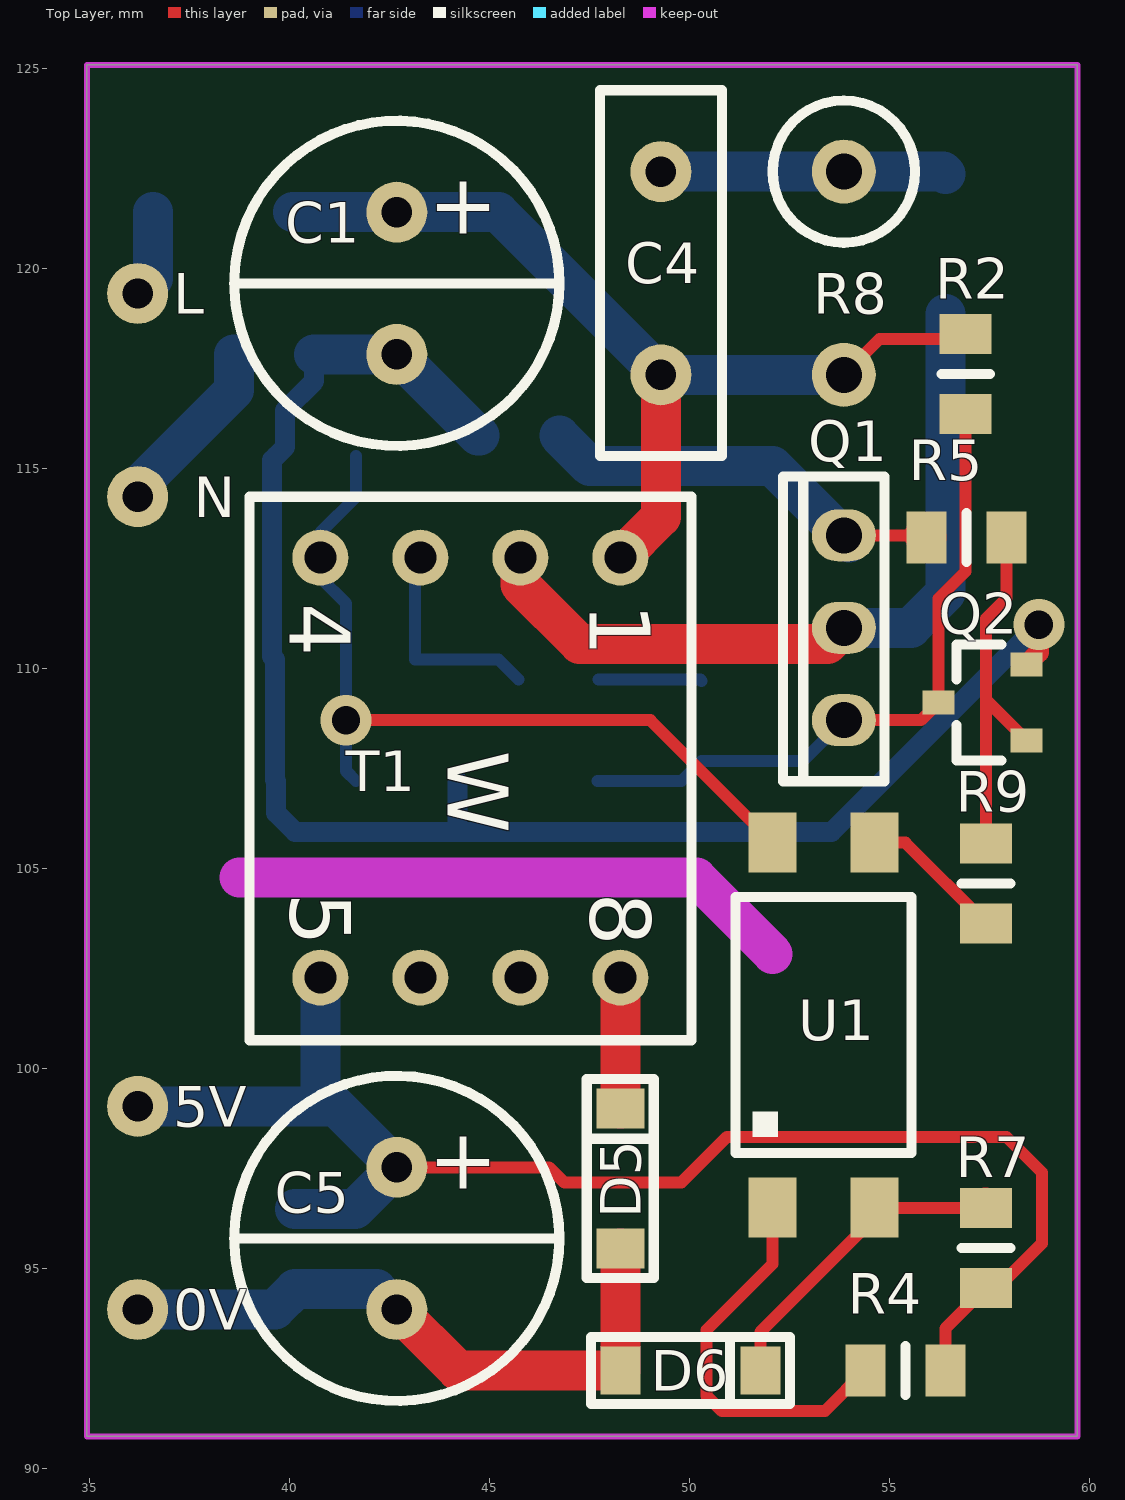
[diagram p0: Top Layer view]
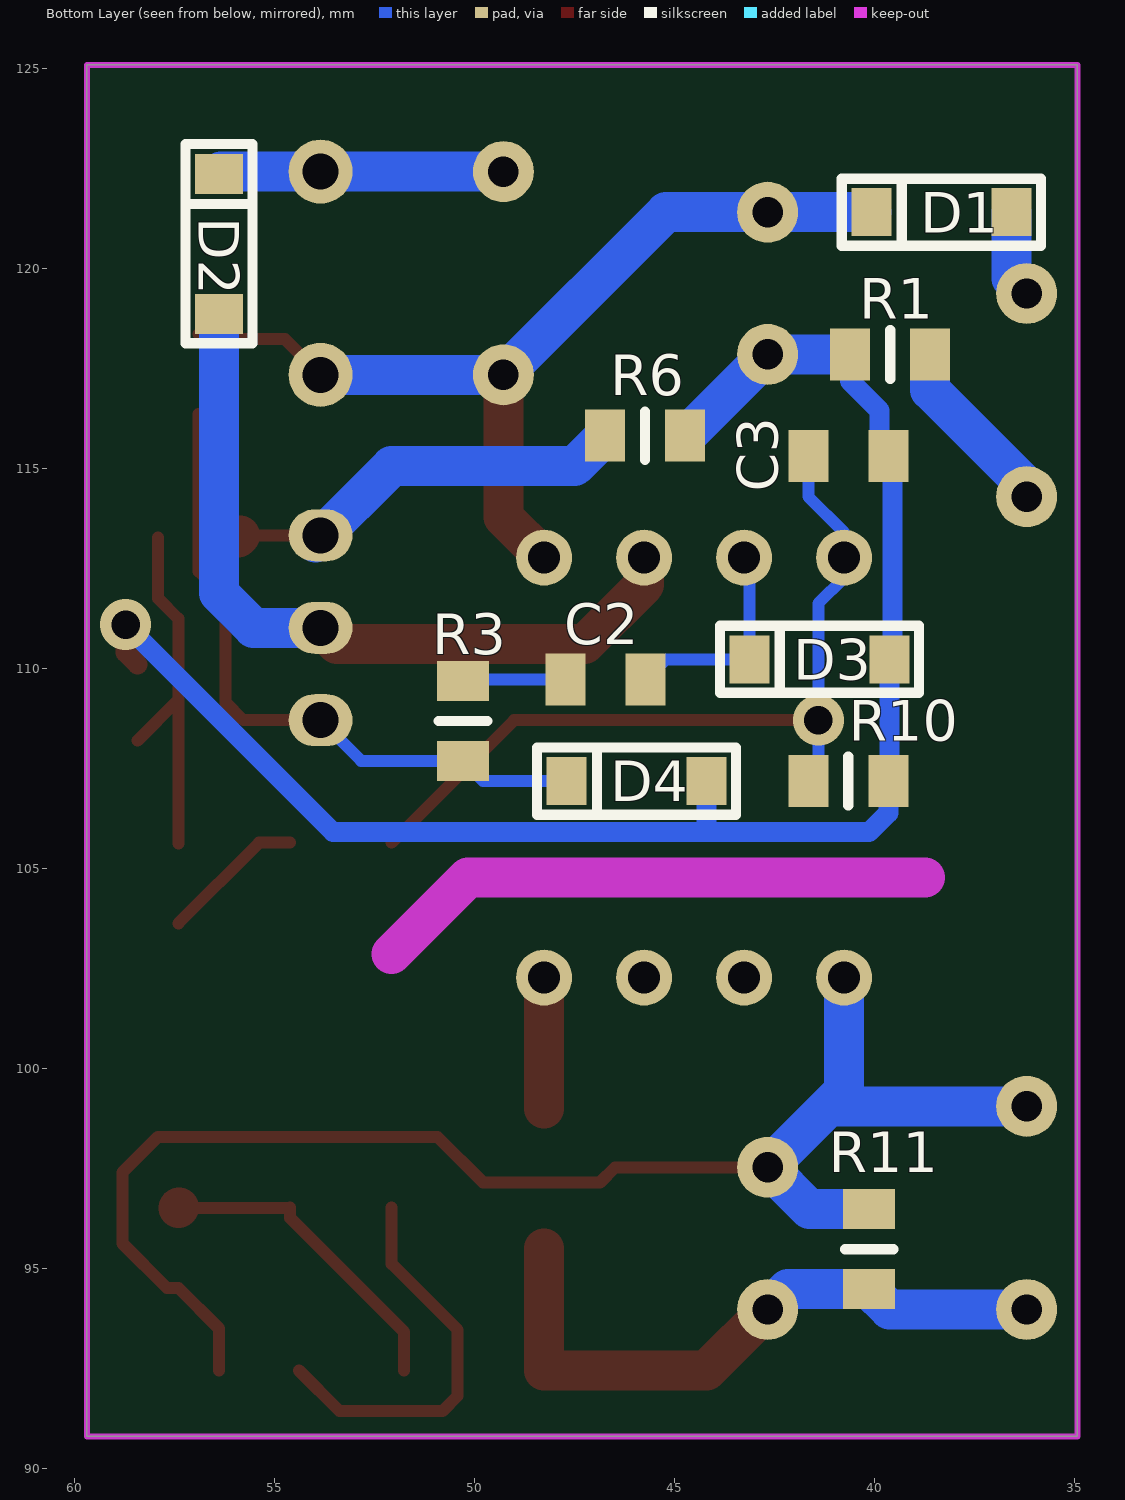
[diagram p1: Bottom Layer view, seen from below]
# Altium PCB MISC95139.PcbDoc
Units mm, origin at the board's own origin, x right, y up, seen from the top; angles counter-clockwise.
Board outline 24.77 x 34.29 mm, 2 copper layers (Top Layer, Bottom Layer); 26 components, 18 nets, 66 pads, 2 vias.

## Layer stack, top to bottom (the 12.6 mil dielectric is the usual default, probably not edited)
Top Layer: signal copper 0.0356
Dielectric: dielectric 0.32, FR-4, Dk 4.8
Bottom Layer: signal copper 0.0356

## Board outline
34.925,125.095 34.925,90.805 59.69,90.805 59.69,125.095

## Design rules (kind name [scope] priority, off if disabled: settings)
Clearance [All] p1: gap=0.254
PolygonConnect [All] p1: connectstyle=Relief reliefconductorwidth=0.254 reliefentries=4 polygonreliefangle="90 Angle"
RoutingVias [All] p1: holewidth=0.711 width=1.27 viastyle="Through Hole" minholewidth=0.711 minwidth=1.27 maxholewidth=0.711 maxwidth=1.27
SilkscreenOverComponentPads [All] p1: minsilkscreentomaskgap=0.254
SolderMaskExpansion [All] p1: expansion=0.102
Width [All] p1: maxlimit=1.5 minlimit=0.3 preferedwidth=1 minimp=50.000000 maximp=50.000000 favimp=50.000000
27 further rules are at their usual default settings.

## Components (designator, comment, footprint, x,y, rotation, side; value= is the part's Value field where it differs from the comment)
C1 "400V4.7uF" cap-8*14mm 42.672,121.412 r270 top
C2 "10nF" 0805_Cap 45.72,109.728 r0 bottom
C3 "16V10uF" 0805_Cap 41.656,115.316 r180 bottom
C4 "1KV4.7nF" CAP_5mm 49.276,117.348 r90 top
C5 "16V470uF" cap-8*14mm 42.672,97.536 r270 top
D1 "1N4007" SOD-123 36.576,121.412 r0 bottom
D2 "FR107" SOD-123 56.388,118.872 r90 bottom
D3 "1N4148" SOD-123 39.624,110.236 r0 bottom
D4 "18V" SOD-123 44.196,107.188 r0 bottom
D5 "B5819W" SOD-123 48.26,95.504 r90 top
D6 "3.9V" SOD-123 48.26,92.456 r0 top
Q1 "1N60" TO-126 53.848,108.712 r90 top
Q2 "J3" SOT23 58.42,108.204 r90 top
R1 "10R" 0805_Res 38.608,117.856 r0 bottom
R2 "2.2M" 0805_Res 56.896,118.364 r270 top
R3 "1K" 0805_Res 50.292,107.696 r90 bottom
R4 "10R" 0805_Res 56.388,92.456 r180 top
R5 "200R" 0805_Res 57.912,113.284 r180 top
R6 "4.7R" 0805_Res 46.736,115.824 r180 bottom
R7 "200R" 0805_Res 57.404,96.52 r270 top
R8 "82K/1W" 1W_Res_L 53.848,122.428 r270 top
R9 "200R" 0805_Res 57.404,103.632 r90 top
R10 "10K" 0805_Res 41.656,107.188 r180 bottom
R11 "1K" 0805_Res 40.132,94.488 r90 bottom
T1 "EE10_4+4_W" EE10_4+4_W 48.26,112.776 r270 top
U1 "PC817" SOP4-PC817 53.34,101.092 r90 top

## Footprints (in the part's own frame and the unit in brackets; to place one, negate y for a bottom-side part, rotate by r counter-clockwise, add the part's x,y. Pads: shape width x height; smd on the part's side, far side on the other; paste and mask are expansions set on the pad)
1W_Res_L [mm]
  round 1.6 hole 0.9: 1(5.08,0) 2(0,0)
  silkscreen extent -1.78,-1.78 1.78,1.78
0805_Cap [mm]
  rect 1x1.3 smd: 1(0,0) 2(2,0)
0805_Res [mm]
  rect 1x1.3 smd: 1(0,0) 2(2,0)
  silkscreen extent 1,-0.61 1,0.61
cap-8*14mm [mil] "470uF/16V,diameter_8mm,height_14mm"
  round 60 hole 30: 1(0,0) 2(140,0)
  silkscreen extent -90,-160 230,160
CAP_5mm [mil] "10nF/1KV,Pin Distance 5mm"
  round 60 hole 30: 1(0,0) 2(200,0)
  silkscreen extent -80,-60 280,60
EE10_4+4_W [mm]
  round 1.4 hole 0.8: 1(0,0) 2(0,-2.5) 3(0,-5) 4(0,-7.5) 5(10.5,-7.5) 6(10.5,-5) 7(10.5,-2.5) 8(10.5,0)
  silkscreen extent -1.52,-9.27 12.07,1.78
SOD-123 [mm]
  rect 1x1.2 smd: 1(0,0) 2(3.5,0)
  silkscreen extent -0.74,-0.84 4.24,0.84
SOP4-PC817 [mm] "SOP4 for PC817"
  rect 1.5x1.2 smd: 1(-4.56,1.27) 2(-4.56,-1.27) 3(4.56,-1.27) 4(4.56,1.27)
  silkscreen extent -3.2,-2.2 3.2,2.2
SOT23 [mm]
  rect 0.6x0.8 smd: 1(0,0) 2(1.9,0) 3(0.95,2.2)
  silkscreen extent -0.5,0.64 2.4,1.75
TO-126 [mm]
  oval 1.3x1.6 hole 0.9: 1(0,0) 2(2.311,0) 3(4.623,0)
  silkscreen extent -1.52,-1.02 6.1,1.52

## Part data
C1 C3 C5: library part "Cap Pol"
C2 C4: library part Cap, "Capacitor"
D1 D2 D3 D5: library part Diode
D4 D6: library part DZener
Q1: library part FQPF20N60C, "600V 20A N-Channel MOSFET"
Q2: "SMD 9013 NPN-Transistor Vceo=25V,Icm=0.5A"
R1 R2 R3 R4 R5 R6 R7 R8 R9 R10 R11: library part Res2, "Resistor"
T1: library part "Flyback transformer-1"
U1: "Device Specification For PhotoCoupler"

## Free pads (board coordinates)
  round 1.524 hole 0.762: 0(36.195,119.38) 1(36.195,114.3) 2(36.195,99.06) 3(36.195,93.98)

## Via types
v1: diameter 1.27, hole 0.711, Top Layer to Bottom Layer, tented both sides, 2 vias

## Nets (pads, with @x,y where several pads share a name; then routed paths per layer and width w, separated by ;. In a path a pad name is that pad's centre, name@x,y a point inside that pad or via, vN(x,y) a via of type N, cw(c..) or ccw(c..) an arc to the next point about the centre after c; other vN are vias at no path point)
+5V: C5.1 pad.2 R4.1 R7.2 R11.2 T1.5 | length 36.7
  Top Layer w0.3: C5.1 46.482,97.536 46.863,97.155 49.784,97.155 50.927,98.298 57.912,98.298 58.801,97.409 58.801,95.631 57.69,94.52 R7.2 56.388,93.504 R4.1
  Bottom Layer w1: pad.2 41.148,99.06 ; R11.2 41.624,96.488 C5.1 41.148,99.06 ; T1.5 40.76,99.448 41.148,99.06
GND: C5.2 D5.1 D6.1 pad.3 R11.1 | length 16.2
  Top Layer w1: C5.2 44.196,92.456 D6.1 D5.1
  Bottom Layer w1: pad.3 39.624,93.98 R11.1 42.164,94.488 C5.2
HGND: C1.2 C3.2 D3.1 D4.1 Q2.2 R1.2 R6.2 R10.2 | length 40.7
  Top Layer w0.5: Q2.2 58.724,110.408 v1(58.724,111.103)
  Bottom Layer w0.3: R10.2@39.624,107.188 R10.2@39.624,107.22
  Bottom Layer w0.5: R10.2@39.624,107.22 D3.1 39.556,110.304 39.556,115.216 C3.2 39.878,115.538 39.878,116.459 40.608,117.189 R1.2 ; R10.2 39.656,106.394 40.132,105.918 44.196,105.918 ; D4.1 44.196,105.918 ; v1(58.724,111.103) 53.539,105.918 44.196,105.918
  Bottom Layer w1: R1.2 C1.2 44.704,115.824 R6.2
L: D1.1 pad.0 | length 2.2
  Bottom Layer w1: pad.0 36.576,119.761 D1.1
N: pad.1 R1.1 | length 4.6
  Bottom Layer w1: pad.1 36.195,114.554 38.608,116.967 R1.1
NetC1_1: C1.1 C4.1 D1.2 R2.1 R8.1 T1.1 | length 23.9
  Top Layer w0.3: R8.1 54.737,118.237 56.769,118.237 R2.1
  Top Layer w1: T1.1 49.276,113.792 C4.1
  Bottom Layer w1: D1.2 C1.1 45.212,121.412 C4.1 R8.1
NetC2_1: C2.1 D3.2 T1.3 | length 5.4
  Bottom Layer w0.3: T1.3 43.124,112.64 D3.2 45.212,110.236 C2.1
NetC2_2: C2.2 R3.2 | length 2.6
  Bottom Layer w0.3: C2.2 50.26,109.728 R3.2
NetC3_1: C3.1 R10.1 T1.4 U1.4 | length 20.8
  Top Layer w0.3: v1(41.402,108.712) 49.01,108.712 U1.4
  Bottom Layer w0.3: R10.1 41.402,107.442 41.402,111.633 40.76,112.275 T1.4 40.76,113.404 41.656,114.3 C3.1
NetC4_2: C4.2 D2.2 R8.2 | length 7.1
  Bottom Layer w1: C4.2 R8.2 56.332,122.428 D2.2
NetD2_1: D2.1 Q1.2 T1.2 | length 19.4
  Top Layer w1: T1.2 45.76,112.101 47.244,110.617 53.442,110.617 Q1.2
  Bottom Layer w1: Q1.2 55.524,111.023 56.388,111.887 D2.1
NetD4_2: D4.2 Q1.1 Q2.3 R2.2 R3.1 | length 16.8
  Top Layer w0.3: Q1.1 55.778,108.712 Q2.3 56.22,111.76 56.896,112.436 R2.2
  Bottom Layer w0.3: D4.2 49.784,107.188 R3.1 52.832,107.696 Q1.1
NetD5_2: D5.2 T1.8 | length 3.3
  Top Layer w1: D5.2 T1.8
NetD6_2: D6.2 R7.1 U1.2 | length 8.1
  Top Layer w0.3: D6.2 51.76,93.416 54.61,96.266 U1.2 ; U1.2@54.622,96.52 R7.1
  Top Layer w1: R7.1@57.392,96.532 R7.1
NetQ1_3: Q1.3 R5.2 R6.1 | length 10.4
  Top Layer w0.3: Q1.3 R5.2@55.861,113.335
  Top Layer w1: R5.2@55.861,113.335 R5.2
  Bottom Layer w1: R6.1 47.498,115.062 52.07,115.062 Q1.3@53.975,113.157
NetQ2_1: Q2.1 R5.1 R9.2 | length 9.3
  Top Layer w0.3: R9.2 57.404,109.22 ; R5.1 57.912,111.76 57.404,111.252 57.404,109.22 ; Q2.1 57.404,109.22
NetR4_2: R4.2 U1.1 | length 9.9
  Top Layer w0.3: U1.1 52.07,95.123 50.419,93.472 50.419,91.821 50.8,91.44 53.372,91.44 R4.2
NetR9_1: R9.1 U1.3 | length 3.6
  Top Layer w0.3: U1.3 55.384,105.652 R9.1
pads on no net: T1.6 T1.7

## Keep-outs
Keep-Out Layer:
  lines w0.154: 34.925,90.805 59.69,90.805 59.69,125.095 34.925,125.095 34.925,90.805
  lines w1: 38.735,104.775 50.165,104.775 52.07,102.87

## Silkscreen, mask and mechanical layers (free items; w line width, h text height)
Top Overlay:
  text "L" at 37.084,118.872 h1.02
  text "N" at 37.592,113.792 h1.02
  text "5V" at 37.084,98.552 h1.02
  text "0V" at 37.084,93.472 h1.02